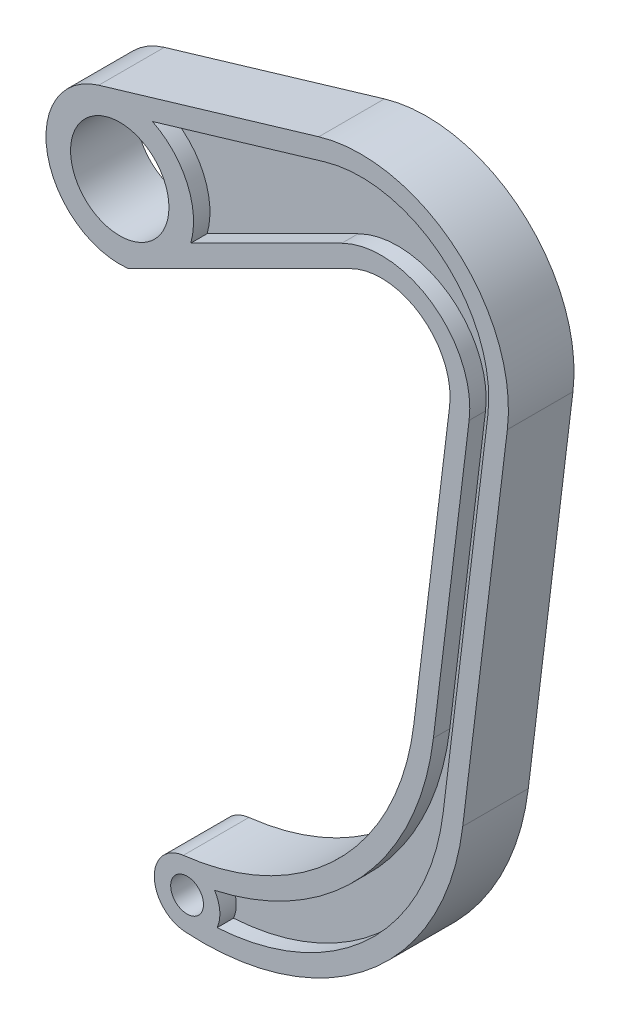
from build123d import *

# Parameters (mm, degrees)
BOSS_EXTRUDE1_DEPTH = 10
BOSS_EXTRUDE2_DEPTH = 20


with BuildPart() as part:
    # Sketch2 → Boss-Extrude1 (new body)
    with BuildSketch(Plane.XY):
        with BuildLine():
            Line((618.099915724, 106.517812479), (565.662842819, 90.936888582))
            ThreePointArc((565.662842819, 90.936888582), (576.256823377, 79.908186522), (577.354047602, 64.654964167))
            Line((577.354047602, 64.654964167), (623.40627245, 87.664511809))
            ThreePointArc((623.40627245, 87.664511809), (651.001261382, 85.576828369), (662.223491353, 60.280516566))
            Line((662.223491353, 60.280516566), (651.330966137, -29.057901231))
            ThreePointArc((651.330966137, -29.057901231), (629.656554116, -76.434863517), (584.606448191, -102.60440016))
            ThreePointArc((584.606448191, -102.60440016), (586.193547668, -107.242337985), (585.385803247, -112.077304476))
            ThreePointArc((585.385803247, -112.077304476), (631.589727703, -92.09112966), (654.31659075, -47.171874157))
            Line((654.31659075, -47.171874157), (667.921518172, 64.413150063))
            ThreePointArc((667.921518172, 64.413150063), (654.381801444, 98.92065746), (618.099915724, 106.517812479))
        make_face()
    extrude(amount=-BOSS_EXTRUDE1_DEPTH)

    # Sketch3 → Boss-Extrude2 (add)
    with BuildSketch(Plane.XY.offset(5)):
        with BuildLine():
            Line((616.390948328, 112.269284503), (549.290441383, 92.331331557))
            ThreePointArc((549.290441383, 92.331331557), (533.654573144, 66.258847309), (558.265088008, 48.410111539))
            Line((558.265088008, 48.410111539), (626.088009426, 82.297176642))
            ThreePointArc((626.088009426, 82.297176642), (647.542544399, 80.674045809), (656.267596834, 61.006684914))
            Line((656.267596834, 61.006684914), (645.375071617, -28.331732883))
            ThreePointArc((645.375071617, -28.331732883), (622.332456349, -75.416562354), (575.086767417, -98.127532436))
            ThreePointArc((575.086767417, -98.127532436), (566.230106721, -108.302539786), (575.565314818, -118.040357973))
            ThreePointArc((575.565314818, -118.040357973), (631.883168962, -99.833110413), (660.27248527, -47.898042505))
            Line((660.27248527, -47.898042505), (673.877412692, 63.686981716))
            ThreePointArc((673.877412692, 63.686981716), (658.254662621, 103.503336404), (616.390948328, 112.269284503))
        make_face()
        with BuildLine():
            ThreePointArc((618.099915724, 106.517812479), (654.381801444, 98.92065746), (667.921518172, 64.413150063))
            Line((667.921518172, 64.413150063), (654.31659075, -47.171874157))
            ThreePointArc((654.31659075, -47.171874157), (631.589727703, -92.09112966), (585.385803247, -112.077304476))
            ThreePointArc((585.385803247, -112.077304476), (586.193547668, -107.242337985), (584.606448191, -102.60440016))
            ThreePointArc((584.606448191, -102.60440016), (629.656554116, -76.434863517), (651.330966137, -29.057901231))
            Line((651.330966137, -29.057901231), (662.223491353, 60.280516566))
            ThreePointArc((662.223491353, 60.280516566), (651.001261382, 85.576828369), (623.40627245, 87.664511809))
            Line((623.40627245, 87.664511809), (577.354047602, 64.654964167))
            ThreePointArc((577.354047602, 64.654964167), (576.256823377, 79.908186522), (565.662842819, 90.936888582))
            Line((565.662842819, 90.936888582), (618.099915724, 106.517812479))
        make_face(mode=Mode.SUBTRACT)
        with BuildLine():
            ThreePointArc((557.409748377, 55.861178182), (540.79693583, 69.052632206), (553.988389854, 85.665444753))
            ThreePointArc((553.988389854, 85.665444753), (570.601202401, 72.47399073), (557.409748377, 55.861178182))
        make_face(mode=Mode.SUBTRACT)
        with BuildLine():
            ThreePointArc((576.797446678, -113.029665722), (571.259842496, -108.632514381), (575.656993837, -103.094910198))
            ThreePointArc((575.656993837, -103.094910198), (581.19459802, -107.492061539), (576.797446678, -113.029665722))
        make_face(mode=Mode.SUBTRACT)
    extrude(amount=-BOSS_EXTRUDE2_DEPTH)


solid = part.part
